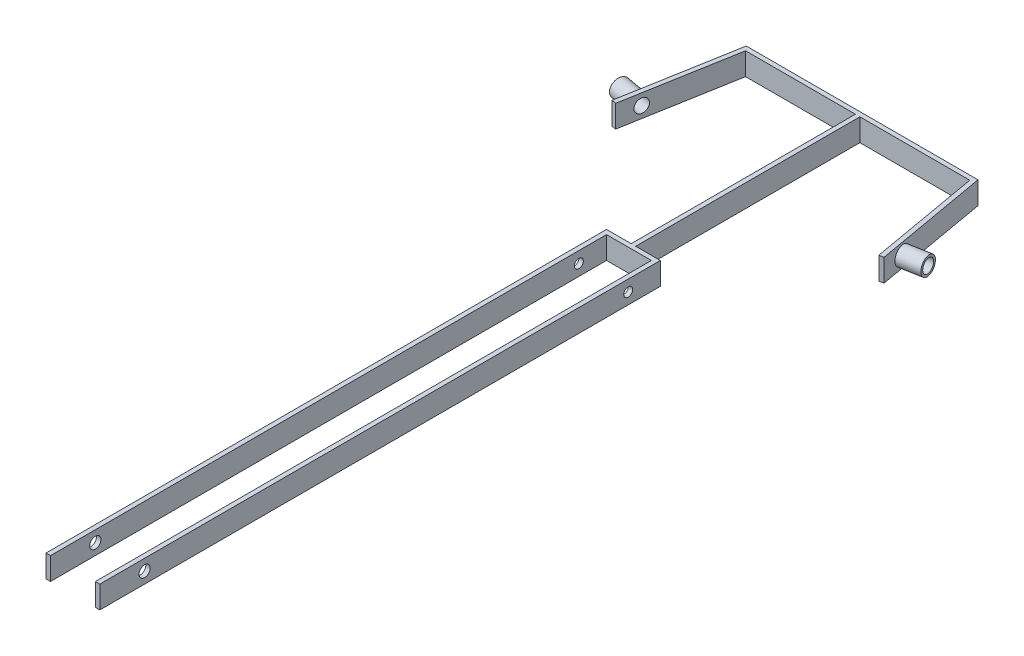
SolidWorks part; units mm, degrees
ref_plane "前视基准面" through (0, 0, 0) normal (0, 0, 1) x (1, 0, 0)
ref_plane "上视基准面" through (0, 0, 0) normal (0, 1, 0) x (1, 0, 0)
ref_plane "右视基准面" through (0, 0, 0) normal (1, 0, 0) x (0, 0, -1)
sketch "草图1" plane through (0, 0, 0) normal (0, 1, 0) x (1, 0, 0)
  line L0 (-10, -248) -> (-10, 0)
  line L1 (-55, 0) -> (55, 0) construction
  line L2 (-10, 0) -> (10, 0)
  line L3 (10, 0) -> (10, -248)
  line L4 (-12, -248) -> (-12, 2)
  line L5 (-12, 2) -> (12, 2)
  line L6 (12, 2) -> (12, -248)
  line L7 (-12, -248) -> (-10, -248)
  line L8 (10, -248) -> (12, -248)
  point P6 (0, 0)
  dimension "D1" = 20
  dimension "D2" = 2
  dimension "D3" = 250
  dimension "D4" = 250
extrude "凸台-拉伸1" add sketch "草图1" along normal blind 10
sketch "草图3" plane through (0, 0, 0) normal (1, 0, 0) x (0, 0, -1)
  line L0 (2, 10) -> (102, 10)
  line L1 (2, 10) -> (2, 0) construction
  line L2 (102, 10) -> (102, 0)
  line L3 (102, 0) -> (2, 0)
  line L4 (2, 0) -> (2, 10)
  line L5 (-248, 5) -> (46.6333, 5) construction
  line L6 (-248, 10) -> (-248, 0) construction
  dimension "D2" = 100
extrude "凸台-拉伸2" add sketch "草图3" along normal mid plane 2
sketch "草图4" plane through (0, 0, 0) normal (0, 1, 0) x (1, 0, 0)
  line L0 (-50, 102) -> (50, 102)
  line L1 (50, 102) -> (58.6824, 52.7596)
  line L2 (-50, 102) -> (-58.6824, 52.7596)
  line L3 (0, 138.2835) -> (0, -64.2777) construction
  line L4 (0, -5.5) -> (0, 5.5) construction
  line L5 (12, 2) -> (1, 2) construction
  line L6 (51.6782, 104) -> (60.652, 53.1069)
  line L7 (-51.6782, 104) -> (51.6782, 104)
  line L8 (-51.6782, 104) -> (-60.652, 53.1069)
  line L9 (-58.6824, 52.7596) -> (-60.652, 53.1069)
  line L10 (60.652, 53.1069) -> (58.6824, 52.7596)
  dimension "D1" = 100
  dimension "D2" = 100
  dimension "D3" = 100
  dimension "D4" = 50
  dimension "D5" = 50
  dimension "D6" = 100
  dimension "D7" = 2
extrude "凸台-拉伸3" add sketch "草图4" along normal blind 10
sketch "草图6" plane through (-67.905, 0, -11.9735) normal (-0.9848, 0, -0.1736) x (-0.1736, 0, 0.9848)
  line L0 (-41.768, 10) -> (-41.768, 0) construction
  circle A0 centre (-51.768, 5) radius 4
  circle A1 centre (-51.768, 5) radius 3
  dimension "D2" = 8
  dimension "D3" = 6
  dimension "D1" = 10
extrude "凸台-拉伸4" add sketch "草图6" along normal blind 10
sketch "草图7" plane through (-67.905, 0, -11.9735) normal (-0.9848, 0, -0.1736) x (-0.1736, 0, 0.9848)
  circle A0 centre (-51.768, 5) radius 3
extrude "切除-拉伸1" cut sketch "草图7" against normal blind 20
mirror "镜向1" about plane through (0, 0, 0) normal (1, 0, 0) of "凸台-拉伸4", "切除-拉伸1"
sketch "草图9" plane through (-12, 0, 0) normal (-1, 0, 0) x (0, 0, 1)
  line L0 (248, 10) -> (248, 0) construction
  circle A0 centre (228, 5) radius 2.5
  dimension "D1" = 5
  dimension "D2" = 20
extrude "切除-拉伸2" cut sketch "草图9" against normal blind 274
sketch "草图10" plane through (-12, 0, 0) normal (-1, 0, 0) x (0, 0, 1)
  circle A0 centre (12.3391, 5) radius 2
  dimension "D1" = 4
extrude "切除-拉伸3" cut sketch "草图10" against normal blind 45
